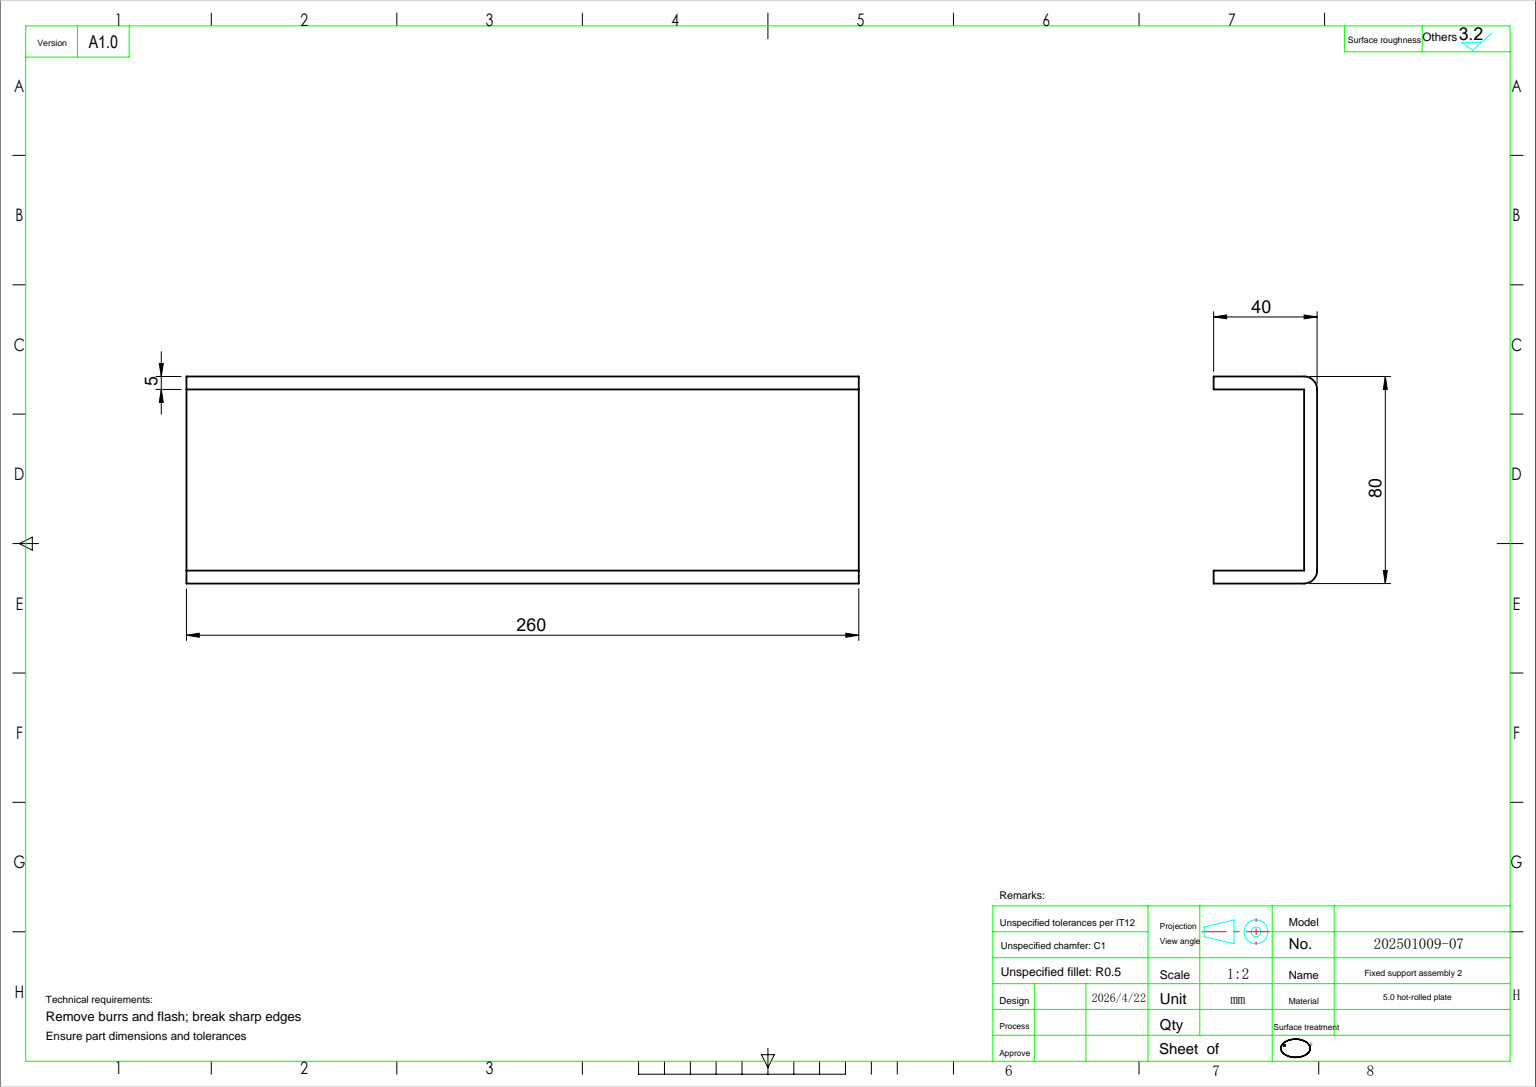
SolidWorks part; units mm, degrees
ref_plane "前视基准面" through (0, 0, 0) normal (0, 0, 1) x (1, 0, 0)
ref_plane "上视基准面" through (0, 0, 0) normal (0, 1, 0) x (1, 0, 0)
ref_plane "右视基准面" through (0, 0, 0) normal (1, 0, 0) x (0, 0, -1)
sketch "草图1" plane through (0, 0, 0) normal (0, 0, 1) x (1, 0, 0)
  line L0 (0, 40) -> (0, -40)
  line L1 (0, -40) -> (40, -40)
  line L2 (0, 40) -> (40, 40)
  dimension "D1" = 80
  dimension "D2" = 40
extrude "拉伸-薄壁1" add sketch "草图1" along normal blind 260 thin thin type one direction wall 5
fillet "圆角1" radius 5 2 edges at (0, -40, 130) (0, 40, 130)
